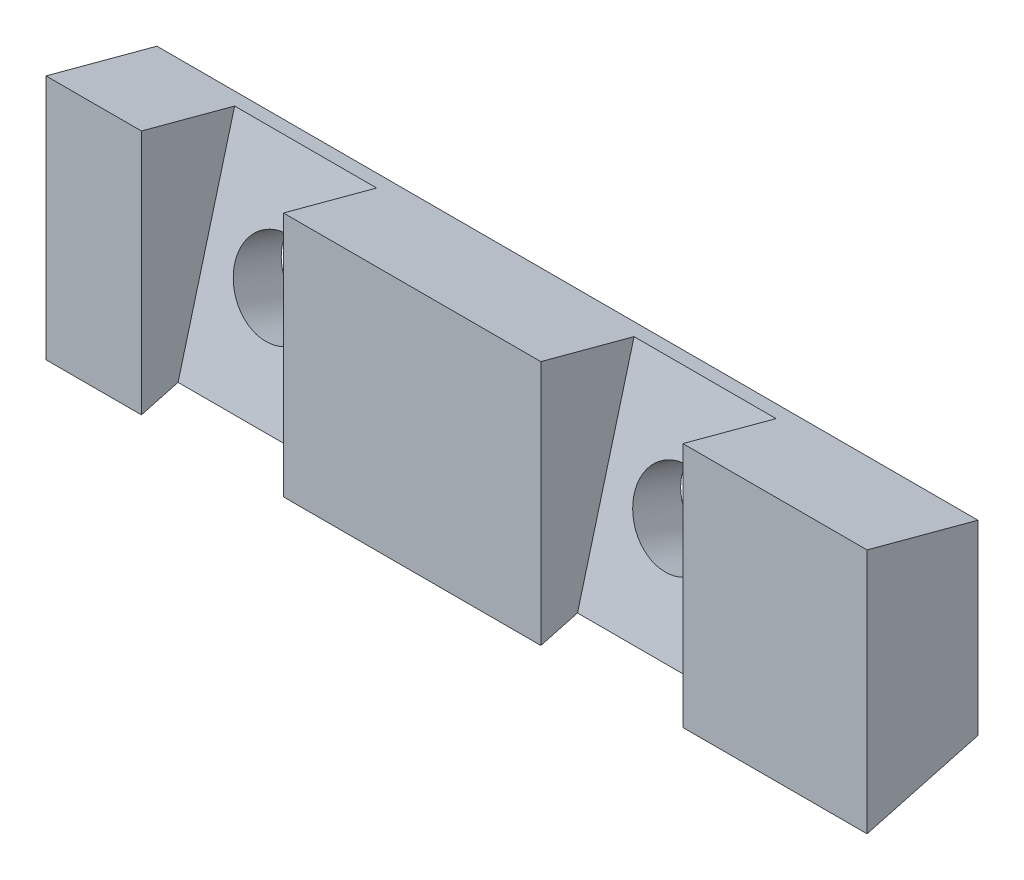
from build123d import *

# Parameters (mm, degrees)
BOSS_EXTRUDE1_DEPTH = 185
BOSS_EXTRUDE2_DEPTH = 35
CUT_EXTRUDE1_START  = -110
CUT_EXTRUDE1_DEPTH  = 32
CUT_EXTRUDE2_START  = 70
CUT_EXTRUDE2_DEPTH  = 32
SKETCH6_W           = 76.501144457
SKETCH6_H           = 19
LPATTERN1_COUNT     = 2
LPATTERN1_PITCH     = 180


with BuildPart() as part:
    # Sketch1 → Boss-Extrude1 (new, symmetric)
    with BuildSketch(Plane(origin=(0, 0, 0), x_dir=(0, 0, -1), z_dir=(1, 0, 0))):
        Polygon((0, 0), (0, 110.794919243), (50, 97.397459622), (50, 13.397459622), align=None)
    extrude(amount=BOSS_EXTRUDE1_DEPTH, both=True)

    # Sketch2 → Boss-Extrude2 (add)
    with BuildSketch(Plane.ZY.offset(185)):
        Polygon((0, 0), (-50, 0), (-50, 13.397459622), align=None)
    extrude(amount=-BOSS_EXTRUDE2_DEPTH)

    # Sketch3 → Cut-Extrude1 (cut, symmetric)
    with BuildSketch(Plane(origin=(0, 0, 0), x_dir=(0, 0, -1), z_dir=(1, 0, 0)).offset(CUT_EXTRUDE1_START)):
        Polygon((16.51733163, 4.425805671), (42.003158605, 99.540206815), (0, 110.794919243), (0, 0), align=None)
    extrude(amount=CUT_EXTRUDE1_DEPTH, both=True, mode=Mode.SUBTRACT)

    # Sketch4 → Cut-Extrude2 (cut, symmetric)
    with BuildSketch(Plane(origin=(0, 0, 0), x_dir=(0, 0, -1), z_dir=(1, 0, 0)).offset(CUT_EXTRUDE2_START)):
        Polygon((16.51733163, 4.425805671), (42.003158605, 99.540206815), (0, 110.794919243), (0, 0), align=None)
    extrude(amount=CUT_EXTRUDE2_DEPTH, both=True, mode=Mode.SUBTRACT)

    # Sketch6 → Cut-Revolve1 (revolve, cut)
    with BuildSketch(Plane(origin=(0, 54.390611447, -19.79656359), x_dir=(0, 0.342020143325663, 0.9396926207859105), z_dir=(0, 0.9396926207859105, -0.342020143325663)), mode=Mode.PRIVATE) as cut_revolve1_sk:
        with Locations((-25.35224184, -100.5)):
            Rectangle(SKETCH6_W, SKETCH6_H)
    cut_revolve1 = revolve(cut_revolve1_sk.sketch.rotate(Axis((-110, 31.16565465, -83.606607958), (0, 0.342020143325663, 0.9396926207859105)), 270), axis=Axis((-110, 31.16565465, -83.606607958), (0, 0.342020143325663, 0.9396926207859105)), mode=Mode.SUBTRACT)

    # LPattern1: Cut-Revolve1 ×2
    with Locations(*[(i * LPATTERN1_PITCH, 0, 0) for i in range(1, LPATTERN1_COUNT)]):
        add(cut_revolve1, mode=Mode.SUBTRACT)


solid = part.part
